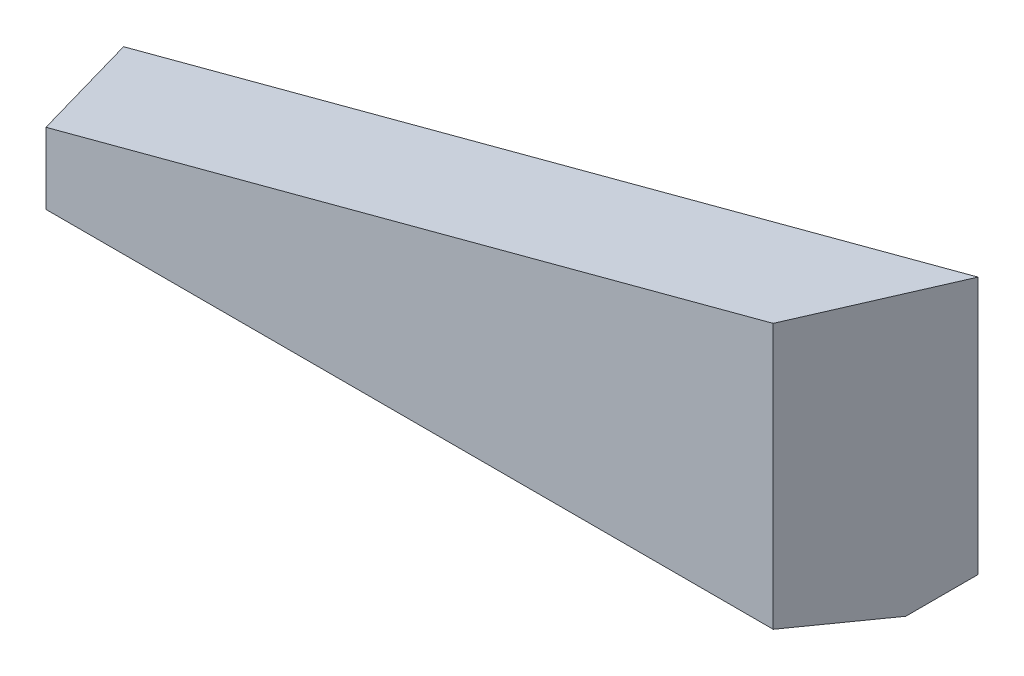
from build123d import *

# Parameters (mm, degrees)
BOSS_EXTRUDE1_DEPTH = 20
CUT_EXTRUDE1_DEPTH  = 50


with BuildPart() as part:
    # Sketch1 → Boss-Extrude1 (new body)
    with BuildSketch(Plane.XY):
        Polygon((5, 0), (137.6, 0), (142.6, 5), (142.6, 48), (0, 10), (0, 5), align=None)
    extrude(amount=BOSS_EXTRUDE1_DEPTH)

    # Sketch2 → Cut-Extrude1 (cut, along a direction that is not the sketch's normal)
    with BuildSketch(Plane(origin=(-2.488112271, 9.33696868, 0), x_dir=(0.9662799118048497, 0.25749394564224604, 0), z_dir=(-0.257493945642246, 0.9662799118048496, 0))):
        Polygon((150.151224814, 0), (135.474939456, -20), (150.151224814, -20), align=None)
        Polygon((2.574939456, -20), (2.574939456, 0), (9.874939456, -20), align=None)
    extrude(amount=-CUT_EXTRUDE1_DEPTH, dir=(0, 1, 0), mode=Mode.SUBTRACT)


solid = part.part
